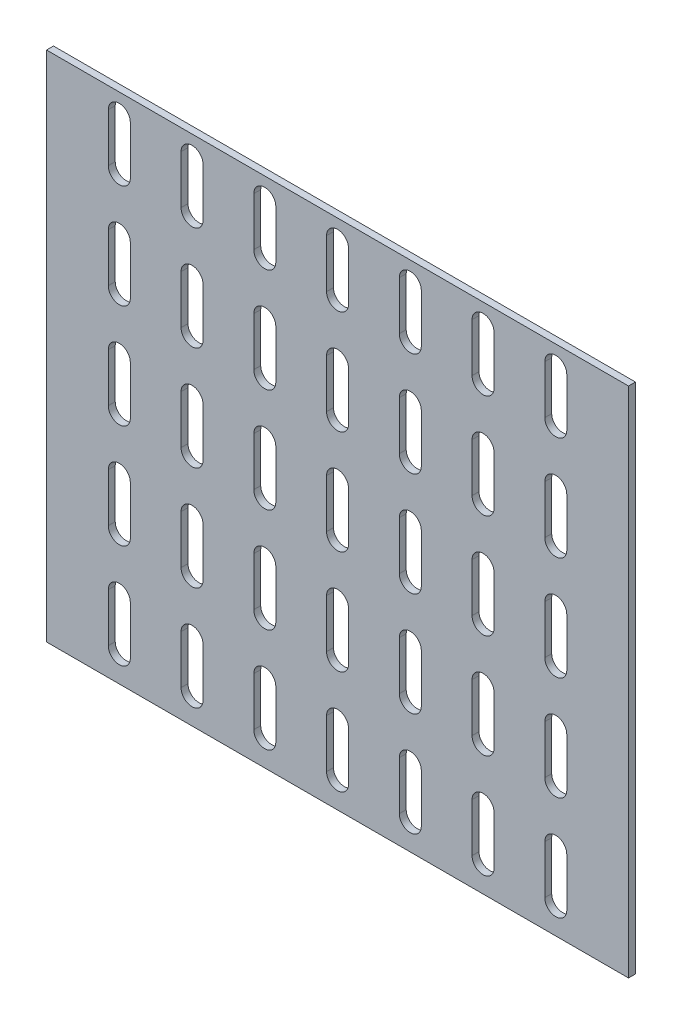
SolidWorks part; units mm, degrees
ref_plane "Front Plane" through (0, 0, 0) normal (0, 0, 1) x (1, 0, 0)
ref_plane "Top Plane" through (0, 0, 0) normal (0, 1, 0) x (1, 0, 0)
ref_plane "Right Plane" through (0, 0, 0) normal (1, 0, 0) x (0, 0, -1)
other "Configuration Table"
sketch "Sketch1" plane through (0, 0, 0) normal (0, 0, 1) x (1, 0, 0)
  line L0 (-51.062, 48.9899) -> (788.938, 48.9899)
  line L1 (788.938, 48.9899) -> (788.938, -691.0101)
  line L2 (788.938, -691.0101) -> (-51.062, -691.0101)
  line L3 (-51.062, -691.0101) -> (-51.062, 48.9899)
extrude "Boss-Extrude1" add sketch "Sketch1" along normal blind 10
sketch "Sketch2" plane through (0, 0, 10) normal (0, 0, 1) x (1, 0, 0)
  line L8 (158.938, 18.9899) -> (158.938, -51.0101) construction
  line L9 (69.8183, 18.9899) -> (69.8183, -51.0101)
  line L10 (38.0577, 18.9899) -> (38.0577, -51.0101)
  line L11 (174.8183, 18.9899) -> (174.8183, -51.0101)
  line L12 (143.0577, 18.9899) -> (143.0577, -51.0101)
  line L13 (263.938, 18.9899) -> (263.938, -51.0101) construction
  line L14 (279.8183, 18.9899) -> (279.8183, -51.0101)
  line L15 (248.0577, 18.9899) -> (248.0577, -51.0101)
  line L16 (368.938, 18.9899) -> (368.938, -51.0101) construction
  line L17 (384.8183, 18.9899) -> (384.8183, -51.0101)
  line L18 (353.0577, 18.9899) -> (353.0577, -51.0101)
  line L19 (473.938, 18.9899) -> (473.938, -51.0101) construction
  line L20 (489.8183, 18.9899) -> (489.8183, -51.0101)
  line L21 (458.0577, 18.9899) -> (458.0577, -51.0101)
  line L22 (578.938, 18.9899) -> (578.938, -51.0101) construction
  line L23 (594.8183, 18.9899) -> (594.8183, -51.0101)
  line L24 (563.0577, 18.9899) -> (563.0577, -51.0101)
  line L25 (683.938, 18.9899) -> (683.938, -51.0101) construction
  line L26 (699.8183, 18.9899) -> (699.8183, -51.0101)
  line L27 (668.0577, 18.9899) -> (668.0577, -51.0101)
  line L28 (53.938, -131.0101) -> (53.938, -201.0101) construction
  line L29 (69.8183, -131.0101) -> (69.8183, -201.0101)
  line L30 (38.0577, -131.0101) -> (38.0577, -201.0101)
  line L31 (158.938, -131.0101) -> (158.938, -201.0101) construction
  line L32 (174.8183, -131.0101) -> (174.8183, -201.0101)
  line L33 (143.0577, -131.0101) -> (143.0577, -201.0101)
  line L34 (263.938, -131.0101) -> (263.938, -201.0101) construction
  line L35 (279.8183, -131.0101) -> (279.8183, -201.0101)
  line L36 (248.0577, -131.0101) -> (248.0577, -201.0101)
  line L37 (368.938, -131.0101) -> (368.938, -201.0101) construction
  line L38 (384.8183, -131.0101) -> (384.8183, -201.0101)
  line L39 (353.0577, -131.0101) -> (353.0577, -201.0101)
  line L40 (473.938, -131.0101) -> (473.938, -201.0101) construction
  line L41 (489.8183, -131.0101) -> (489.8183, -201.0101)
  line L42 (458.0577, -131.0101) -> (458.0577, -201.0101)
  line L43 (578.938, -131.0101) -> (578.938, -201.0101) construction
  line L44 (594.8183, -131.0101) -> (594.8183, -201.0101)
  line L45 (563.0577, -131.0101) -> (563.0577, -201.0101)
  line L46 (683.938, -131.0101) -> (683.938, -201.0101) construction
  line L47 (699.8183, -131.0101) -> (699.8183, -201.0101)
  line L48 (668.0577, -131.0101) -> (668.0577, -201.0101)
  line L49 (53.938, -281.0101) -> (53.938, -351.0101) construction
  line L50 (69.8183, -281.0101) -> (69.8183, -351.0101)
  line L51 (38.0577, -281.0101) -> (38.0577, -351.0101)
  line L52 (158.938, -281.0101) -> (158.938, -351.0101) construction
  line L53 (174.8183, -281.0101) -> (174.8183, -351.0101)
  line L54 (143.0577, -281.0101) -> (143.0577, -351.0101)
  line L55 (263.938, -281.0101) -> (263.938, -351.0101) construction
  line L56 (279.8183, -281.0101) -> (279.8183, -351.0101)
  line L57 (248.0577, -281.0101) -> (248.0577, -351.0101)
  line L58 (368.938, -281.0101) -> (368.938, -351.0101) construction
  line L59 (384.8183, -281.0101) -> (384.8183, -351.0101)
  line L60 (353.0577, -281.0101) -> (353.0577, -351.0101)
  line L61 (473.938, -281.0101) -> (473.938, -351.0101) construction
  line L62 (489.8183, -281.0101) -> (489.8183, -351.0101)
  line L63 (458.0577, -281.0101) -> (458.0577, -351.0101)
  line L64 (578.938, -281.0101) -> (578.938, -351.0101) construction
  line L65 (594.8183, -281.0101) -> (594.8183, -351.0101)
  line L66 (563.0577, -281.0101) -> (563.0577, -351.0101)
  line L67 (683.938, -281.0101) -> (683.938, -351.0101) construction
  line L68 (699.8183, -281.0101) -> (699.8183, -351.0101)
  line L69 (668.0577, -281.0101) -> (668.0577, -351.0101)
  line L70 (53.938, -431.0101) -> (53.938, -501.0101) construction
  line L71 (69.8183, -431.0101) -> (69.8183, -501.0101)
  line L72 (38.0577, -431.0101) -> (38.0577, -501.0101)
  line L73 (158.938, -431.0101) -> (158.938, -501.0101) construction
  line L74 (174.8183, -431.0101) -> (174.8183, -501.0101)
  line L75 (143.0577, -431.0101) -> (143.0577, -501.0101)
  line L76 (263.938, -431.0101) -> (263.938, -501.0101) construction
  line L77 (279.8183, -431.0101) -> (279.8183, -501.0101)
  line L78 (248.0577, -431.0101) -> (248.0577, -501.0101)
  line L79 (368.938, -431.0101) -> (368.938, -501.0101) construction
  line L80 (384.8183, -431.0101) -> (384.8183, -501.0101)
  line L81 (353.0577, -431.0101) -> (353.0577, -501.0101)
  line L82 (473.938, -431.0101) -> (473.938, -501.0101) construction
  line L83 (489.8183, -431.0101) -> (489.8183, -501.0101)
  line L84 (458.0577, -431.0101) -> (458.0577, -501.0101)
  line L85 (578.938, -431.0101) -> (578.938, -501.0101) construction
  line L86 (594.8183, -431.0101) -> (594.8183, -501.0101)
  line L87 (563.0577, -431.0101) -> (563.0577, -501.0101)
  line L88 (683.938, -431.0101) -> (683.938, -501.0101) construction
  line L89 (699.8183, -431.0101) -> (699.8183, -501.0101)
  line L90 (668.0577, -431.0101) -> (668.0577, -501.0101)
  line L91 (53.938, -581.0101) -> (53.938, -651.0101) construction
  line L92 (69.8183, -581.0101) -> (69.8183, -651.0101)
  line L93 (38.0577, -581.0101) -> (38.0577, -651.0101)
  line L94 (158.938, -581.0101) -> (158.938, -651.0101) construction
  line L95 (174.8183, -581.0101) -> (174.8183, -651.0101)
  line L96 (143.0577, -581.0101) -> (143.0577, -651.0101)
  line L97 (263.938, -581.0101) -> (263.938, -651.0101) construction
  line L98 (279.8183, -581.0101) -> (279.8183, -651.0101)
  line L99 (248.0577, -581.0101) -> (248.0577, -651.0101)
  line L100 (368.938, -581.0101) -> (368.938, -651.0101) construction
  line L101 (384.8183, -581.0101) -> (384.8183, -651.0101)
  line L102 (353.0577, -581.0101) -> (353.0577, -651.0101)
  line L103 (473.938, -581.0101) -> (473.938, -651.0101) construction
  line L104 (489.8183, -581.0101) -> (489.8183, -651.0101)
  line L105 (458.0577, -581.0101) -> (458.0577, -651.0101)
  line L106 (578.938, -581.0101) -> (578.938, -651.0101) construction
  line L107 (594.8183, -581.0101) -> (594.8183, -651.0101)
  line L108 (563.0577, -581.0101) -> (563.0577, -651.0101)
  line L109 (683.938, -581.0101) -> (683.938, -651.0101) construction
  line L110 (699.8183, -581.0101) -> (699.8183, -651.0101)
  line L111 (668.0577, -581.0101) -> (668.0577, -651.0101)
  arc A0 (69.8183, 18.9899) -> (38.0577, 18.9899) centre (53.938, 18.9899) ccw
  arc A1 (38.0577, -51.0101) -> (69.8183, -51.0101) centre (53.938, -51.0101) ccw
  arc A2 (174.8183, 18.9899) -> (143.0577, 18.9899) centre (158.938, 18.9899) ccw
  arc A3 (143.0577, -51.0101) -> (174.8183, -51.0101) centre (158.938, -51.0101) ccw
  arc A4 (279.8183, 18.9899) -> (248.0577, 18.9899) centre (263.938, 18.9899) ccw
  arc A5 (248.0577, -51.0101) -> (279.8183, -51.0101) centre (263.938, -51.0101) ccw
  arc A6 (384.8183, 18.9899) -> (353.0577, 18.9899) centre (368.938, 18.9899) ccw
  arc A7 (353.0577, -51.0101) -> (384.8183, -51.0101) centre (368.938, -51.0101) ccw
  arc A8 (489.8183, 18.9899) -> (458.0577, 18.9899) centre (473.938, 18.9899) ccw
  arc A9 (458.0577, -51.0101) -> (489.8183, -51.0101) centre (473.938, -51.0101) ccw
  arc A10 (594.8183, 18.9899) -> (563.0577, 18.9899) centre (578.938, 18.9899) ccw
  arc A11 (563.0577, -51.0101) -> (594.8183, -51.0101) centre (578.938, -51.0101) ccw
  arc A12 (699.8183, 18.9899) -> (668.0577, 18.9899) centre (683.938, 18.9899) ccw
  arc A13 (668.0577, -51.0101) -> (699.8183, -51.0101) centre (683.938, -51.0101) ccw
  arc A14 (69.8183, -131.0101) -> (38.0577, -131.0101) centre (53.938, -131.0101) ccw
  arc A15 (38.0577, -201.0101) -> (69.8183, -201.0101) centre (53.938, -201.0101) ccw
  arc A16 (174.8183, -131.0101) -> (143.0577, -131.0101) centre (158.938, -131.0101) ccw
  arc A17 (143.0577, -201.0101) -> (174.8183, -201.0101) centre (158.938, -201.0101) ccw
  arc A18 (279.8183, -131.0101) -> (248.0577, -131.0101) centre (263.938, -131.0101) ccw
  arc A19 (248.0577, -201.0101) -> (279.8183, -201.0101) centre (263.938, -201.0101) ccw
  arc A20 (384.8183, -131.0101) -> (353.0577, -131.0101) centre (368.938, -131.0101) ccw
  arc A21 (353.0577, -201.0101) -> (384.8183, -201.0101) centre (368.938, -201.0101) ccw
  arc A22 (489.8183, -131.0101) -> (458.0577, -131.0101) centre (473.938, -131.0101) ccw
  arc A23 (458.0577, -201.0101) -> (489.8183, -201.0101) centre (473.938, -201.0101) ccw
  arc A24 (594.8183, -131.0101) -> (563.0577, -131.0101) centre (578.938, -131.0101) ccw
  arc A25 (563.0577, -201.0101) -> (594.8183, -201.0101) centre (578.938, -201.0101) ccw
  arc A26 (699.8183, -131.0101) -> (668.0577, -131.0101) centre (683.938, -131.0101) ccw
  arc A27 (668.0577, -201.0101) -> (699.8183, -201.0101) centre (683.938, -201.0101) ccw
  arc A28 (69.8183, -281.0101) -> (38.0577, -281.0101) centre (53.938, -281.0101) ccw
  arc A29 (38.0577, -351.0101) -> (69.8183, -351.0101) centre (53.938, -351.0101) ccw
  arc A30 (174.8183, -281.0101) -> (143.0577, -281.0101) centre (158.938, -281.0101) ccw
  arc A31 (143.0577, -351.0101) -> (174.8183, -351.0101) centre (158.938, -351.0101) ccw
  arc A32 (279.8183, -281.0101) -> (248.0577, -281.0101) centre (263.938, -281.0101) ccw
  arc A33 (248.0577, -351.0101) -> (279.8183, -351.0101) centre (263.938, -351.0101) ccw
  arc A34 (384.8183, -281.0101) -> (353.0577, -281.0101) centre (368.938, -281.0101) ccw
  arc A35 (353.0577, -351.0101) -> (384.8183, -351.0101) centre (368.938, -351.0101) ccw
  arc A36 (489.8183, -281.0101) -> (458.0577, -281.0101) centre (473.938, -281.0101) ccw
  arc A37 (458.0577, -351.0101) -> (489.8183, -351.0101) centre (473.938, -351.0101) ccw
  arc A38 (594.8183, -281.0101) -> (563.0577, -281.0101) centre (578.938, -281.0101) ccw
  arc A39 (563.0577, -351.0101) -> (594.8183, -351.0101) centre (578.938, -351.0101) ccw
  arc A40 (699.8183, -281.0101) -> (668.0577, -281.0101) centre (683.938, -281.0101) ccw
  arc A41 (668.0577, -351.0101) -> (699.8183, -351.0101) centre (683.938, -351.0101) ccw
  arc A42 (69.8183, -431.0101) -> (38.0577, -431.0101) centre (53.938, -431.0101) ccw
  arc A43 (38.0577, -501.0101) -> (69.8183, -501.0101) centre (53.938, -501.0101) ccw
  arc A44 (174.8183, -431.0101) -> (143.0577, -431.0101) centre (158.938, -431.0101) ccw
  arc A45 (143.0577, -501.0101) -> (174.8183, -501.0101) centre (158.938, -501.0101) ccw
  arc A46 (279.8183, -431.0101) -> (248.0577, -431.0101) centre (263.938, -431.0101) ccw
  arc A47 (248.0577, -501.0101) -> (279.8183, -501.0101) centre (263.938, -501.0101) ccw
  arc A48 (384.8183, -431.0101) -> (353.0577, -431.0101) centre (368.938, -431.0101) ccw
  arc A49 (353.0577, -501.0101) -> (384.8183, -501.0101) centre (368.938, -501.0101) ccw
  arc A50 (489.8183, -431.0101) -> (458.0577, -431.0101) centre (473.938, -431.0101) ccw
  arc A51 (458.0577, -501.0101) -> (489.8183, -501.0101) centre (473.938, -501.0101) ccw
  arc A52 (594.8183, -431.0101) -> (563.0577, -431.0101) centre (578.938, -431.0101) ccw
  arc A53 (563.0577, -501.0101) -> (594.8183, -501.0101) centre (578.938, -501.0101) ccw
  arc A54 (699.8183, -431.0101) -> (668.0577, -431.0101) centre (683.938, -431.0101) ccw
  arc A55 (668.0577, -501.0101) -> (699.8183, -501.0101) centre (683.938, -501.0101) ccw
  arc A56 (69.8183, -581.0101) -> (38.0577, -581.0101) centre (53.938, -581.0101) ccw
  arc A57 (38.0577, -651.0101) -> (69.8183, -651.0101) centre (53.938, -651.0101) ccw
  arc A58 (174.8183, -581.0101) -> (143.0577, -581.0101) centre (158.938, -581.0101) ccw
  arc A59 (143.0577, -651.0101) -> (174.8183, -651.0101) centre (158.938, -651.0101) ccw
  arc A60 (279.8183, -581.0101) -> (248.0577, -581.0101) centre (263.938, -581.0101) ccw
  arc A61 (248.0577, -651.0101) -> (279.8183, -651.0101) centre (263.938, -651.0101) ccw
  arc A62 (384.8183, -581.0101) -> (353.0577, -581.0101) centre (368.938, -581.0101) ccw
  arc A63 (353.0577, -651.0101) -> (384.8183, -651.0101) centre (368.938, -651.0101) ccw
  arc A64 (489.8183, -581.0101) -> (458.0577, -581.0101) centre (473.938, -581.0101) ccw
  arc A65 (458.0577, -651.0101) -> (489.8183, -651.0101) centre (473.938, -651.0101) ccw
  arc A66 (594.8183, -581.0101) -> (563.0577, -581.0101) centre (578.938, -581.0101) ccw
  arc A67 (563.0577, -651.0101) -> (594.8183, -651.0101) centre (578.938, -651.0101) ccw
  arc A68 (699.8183, -581.0101) -> (668.0577, -581.0101) centre (683.938, -581.0101) ccw
  arc A69 (668.0577, -651.0101) -> (699.8183, -651.0101) centre (683.938, -651.0101) ccw
  point P18 (53.938, -16.0101)
  point P25 (158.938, -16.0101)
  point P32 (263.938, -16.0101)
  point P39 (368.938, -16.0101)
  point P46 (473.938, -16.0101)
  point P53 (578.938, -16.0101)
  point P60 (683.938, -16.0101)
  point P67 (53.938, -166.0101)
  point P74 (158.938, -166.0101)
  point P81 (263.938, -166.0101)
  point P88 (368.938, -166.0101)
  point P95 (473.938, -166.0101)
  point P102 (578.938, -166.0101)
  point P109 (683.938, -166.0101)
  point P116 (53.938, -316.0101)
  point P123 (158.938, -316.0101)
  point P130 (263.938, -316.0101)
  point P137 (368.938, -316.0101)
  point P144 (473.938, -316.0101)
  point P151 (578.938, -316.0101)
  point P158 (683.938, -316.0101)
  point P165 (53.938, -466.0101)
  point P172 (158.938, -466.0101)
  point P179 (263.938, -466.0101)
  point P186 (368.938, -466.0101)
  point P193 (473.938, -466.0101)
  point P200 (578.938, -466.0101)
  point P207 (683.938, -466.0101)
  point P214 (53.938, -616.0101)
  point P221 (158.938, -616.0101)
  point P228 (263.938, -616.0101)
  point P235 (368.938, -616.0101)
  point P242 (473.938, -616.0101)
  point P249 (578.938, -616.0101)
  point P256 (683.938, -616.0101)
  dimension "D5" = 5
extrude "Cut-Extrude1" cut sketch "Sketch2" against normal blind 10 contours L10 A1 L9 A0 | L11 A3 L12 A2 | L14 A5 L15 A4 | L17 A7 L18 A6 | L20 A9 L21 A8 | L23 A11 L24 A10 | L26 A13 L27 A12 | L47 A27 L48 A26 | L44 A25 L45 A24 | L41 A23 L42 A22 | L38 A21 L39 A20 | L35 A19 L36 A18 | L32 A17 L33 A16 | L29 A15 L30 A14 | L50 A29 L51 A28 | L53 A31 L54 A30 | L56 A33 L57 A32 | L59 A35 L60 A34 | L62 A37 L63 A36 | L65 A39 L66 A38 | L68 A41 L69 A40 | L71 A43 L72 A42 | L74 A45 L75 A44 | L77 A47 L78 A46 | L80 A49 L81 A48 | L83 A51 L84 A50 | L89 A55 L90 A54 | L86 A53 L87 A52 | L107 A67 L108 A66 | L110 A69 L111 A68 | L104 A65 L105 A64 | L101 A63 L102 A62 | L95 A59 L96 A58 | L98 A61 L99 A60 | L92 A57 L93 A56
